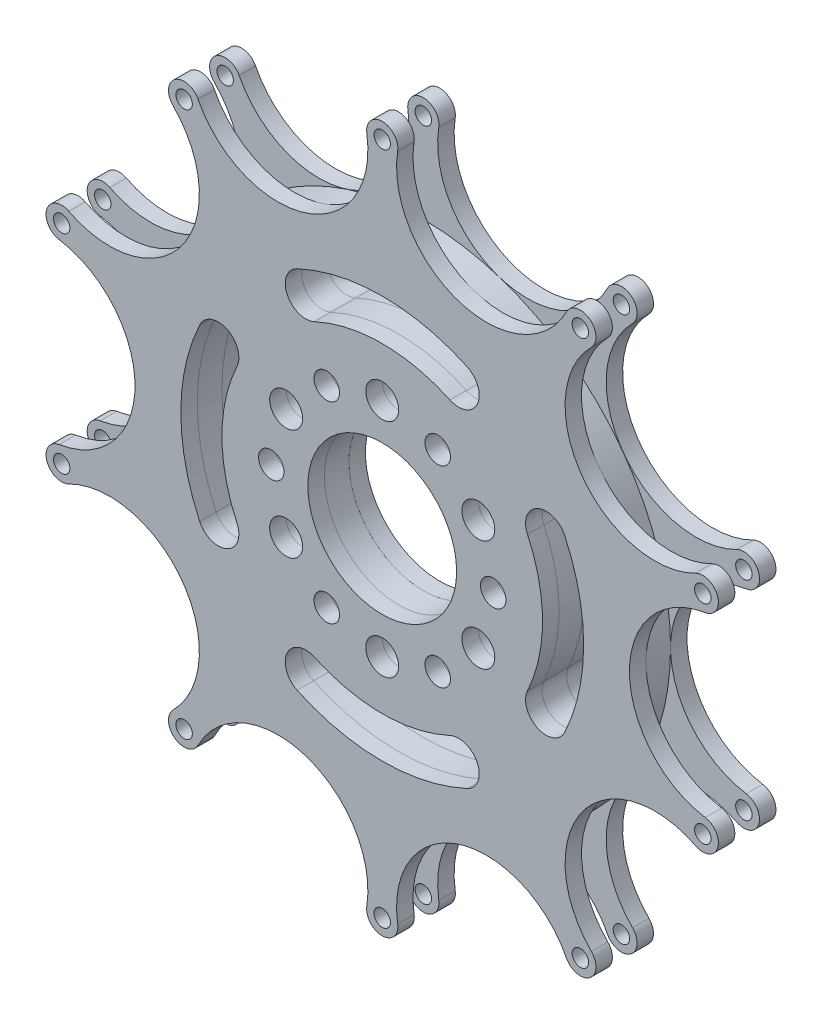
SolidWorks part; units mm, degrees
material "Thornel Mat VMA"
ref_plane "前视基准面" through (0, 0, 0) normal (0, 0, 1) x (1, 0, 0)
ref_plane "上视基准面" through (0, 0, 0) normal (0, 1, 0) x (1, 0, 0)
ref_plane "右视基准面" through (0, 0, 0) normal (1, 0, 0) x (0, 0, -1)
sketch "草图1" plane through (0, 0, 0) normal (0, 0, 1) x (1, 0, 0)
  line L0 (0, 0) -> (0, 41) construction
  circle A0 centre (0, 0) radius 30.0724 construction
  circle A1 centre (0, 0) radius 41 construction
  arc A2 (1.8766, 40.7028) -> (-1.8766, 40.7028) centre (0, 41) ccw
  circle A3 centre (0, 41) radius 1
  arc A4 (1.8766, 40.7028) -> (9.2929, 28.6005) centre (12.6697, 38.9933) ccw
  arc A5 (-1.8766, 40.7028) -> (-9.2929, 28.6005) centre (-12.6697, 38.9933) cw
  circle A6 centre (0, 41) radius 2.5 construction
  arc A7 (25.4427, 31.8262) -> (24.3291, 17.6761) centre (33.1697, 24.0992) ccw
  arc A8 (22.4063, 34.0323) -> (9.2929, 28.6005) centre (12.6697, 38.9933) cw
  arc A9 (25.4427, 31.8262) -> (22.4063, 34.0323) centre (24.0992, 33.1697) ccw
  arc A10 (39.2905, 10.7931) -> (30.0724, 0) centre (41, 0) ccw
  arc A11 (38.1307, 14.3626) -> (24.3291, 17.6761) centre (33.1697, 24.0992) cw
  arc A12 (39.2905, 10.7931) -> (38.1307, 14.3626) centre (38.9933, 12.6697) ccw
  arc A13 (38.1307, -14.3626) -> (24.3291, -17.6761) centre (33.1697, -24.0992) ccw
  arc A14 (39.2905, -10.7931) -> (30.0724, 0) centre (41, 0) cw
  arc A15 (38.1307, -14.3626) -> (39.2905, -10.7931) centre (38.9933, -12.6697) ccw
  arc A16 (22.4063, -34.0323) -> (9.2929, -28.6005) centre (12.6697, -38.9933) ccw
  arc A17 (25.4427, -31.8262) -> (24.3291, -17.6761) centre (33.1697, -24.0992) cw
  arc A18 (22.4063, -34.0323) -> (25.4427, -31.8262) centre (24.0992, -33.1697) ccw
  arc A19 (-1.8766, -40.7028) -> (-9.2929, -28.6005) centre (-12.6697, -38.9933) ccw
  arc A20 (1.8766, -40.7028) -> (9.2929, -28.6005) centre (12.6697, -38.9933) cw
  arc A21 (-1.8766, -40.7028) -> (1.8766, -40.7028) centre (0, -41) ccw
  arc A22 (-25.4427, -31.8262) -> (-24.3291, -17.6761) centre (-33.1697, -24.0992) ccw
  arc A23 (-22.4063, -34.0323) -> (-9.2929, -28.6005) centre (-12.6697, -38.9933) cw
  arc A24 (-25.4427, -31.8262) -> (-22.4063, -34.0323) centre (-24.0992, -33.1697) ccw
  arc A25 (-39.2905, -10.7931) -> (-30.0724, 0) centre (-41, 0) ccw
  arc A26 (-38.1307, -14.3626) -> (-24.3291, -17.6761) centre (-33.1697, -24.0992) cw
  arc A27 (-39.2905, -10.7931) -> (-38.1307, -14.3626) centre (-38.9933, -12.6697) ccw
  arc A28 (-38.1307, 14.3626) -> (-24.3291, 17.6761) centre (-33.1697, 24.0992) ccw
  arc A29 (-39.2905, 10.7931) -> (-30.0724, 0) centre (-41, 0) cw
  arc A30 (-38.1307, 14.3626) -> (-39.2905, 10.7931) centre (-38.9933, 12.6697) ccw
  arc A31 (-22.4063, 34.0323) -> (-9.2929, 28.6005) centre (-12.6697, 38.9933) ccw
  arc A32 (-25.4427, 31.8262) -> (-24.3291, 17.6761) centre (-33.1697, 24.0992) cw
  arc A33 (-22.4063, 34.0323) -> (-25.4427, 31.8262) centre (-24.0992, 33.1697) ccw
  circle A34 centre (-12.6697, 38.9933) radius 9 construction
  circle A36 centre (24.0992, 33.1697) radius 1
  circle A37 centre (38.9933, 12.6697) radius 1
  circle A38 centre (38.9933, -12.6697) radius 1
  circle A39 centre (24.0992, -33.1697) radius 1
  circle A40 centre (0, -41) radius 1
  circle A41 centre (-24.0992, -33.1697) radius 1
  circle A42 centre (-38.9933, -12.6697) radius 1
  circle A43 centre (-38.9933, 12.6697) radius 1
  circle A44 centre (-24.0992, 33.1697) radius 1
  point P78 (0, 0)
  point P88 (0, 0)
  point P98 (0, 0)
  point P107 (0, 0)
  dimension "D1" = 10.9276
  dimension "D2" = 82
  dimension "D3" = 3.8
  dimension "D4" = 2
  dimension "D5" = 5
  dimension "D7" = 60.1447
  dimension "D8" = 18
  dimension "D6" = 10
  dimension "D9" = 10
extrude "凸台-拉伸2" add sketch "草图1" along normal blind 2
sketch "草图2" plane through (0, 0, 2) normal (0, 0, 1) x (1, 0, 0)
  circle A9 centre (0, 0) radius 30.0724 construction
  circle A19 centre (0, 0) radius 30.0724
extrude "凸台-拉伸3" add sketch "草图2" along normal blind 3 separate body
sketch "草图3" plane through (0, 0, 5) normal (0, 0, 1) x (1, 0, 0)
  circle A16 centre (-38.9933, -12.6697) radius 1 construction
  circle A17 centre (-38.9933, 12.6697) radius 1 construction
  circle A18 centre (-24.0992, 33.1697) radius 1 construction
  circle A19 centre (0, 41) radius 1 construction
  arc A20 (-22.4063, 34.0323) -> (-1.8766, 40.7028) centre (-12.6697, 38.9933) ccw
  arc A21 (1.8766, 40.7028) -> (-1.8766, 40.7028) centre (0, 41) ccw
  arc A22 (1.8766, 40.7028) -> (22.4063, 34.0323) centre (12.6697, 38.9933) ccw
  arc A23 (25.4427, 31.8262) -> (22.4063, 34.0323) centre (24.0992, 33.1697) ccw
  arc A24 (25.4427, 31.8262) -> (38.1307, 14.3626) centre (33.1697, 24.0992) ccw
  arc A25 (39.2905, 10.7931) -> (38.1307, 14.3626) centre (38.9933, 12.6697) ccw
  arc A26 (39.2905, 10.7931) -> (39.2905, -10.7931) centre (41, 0) ccw
  arc A27 (38.1307, -14.3626) -> (39.2905, -10.7931) centre (38.9933, -12.6697) ccw
  arc A28 (38.1307, -14.3626) -> (25.4427, -31.8262) centre (33.1697, -24.0992) ccw
  arc A29 (22.4063, -34.0323) -> (25.4427, -31.8262) centre (24.0992, -33.1697) ccw
  arc A30 (22.4063, -34.0323) -> (1.8766, -40.7028) centre (12.6697, -38.9933) ccw
  arc A31 (-1.8766, -40.7028) -> (1.8766, -40.7028) centre (0, -41) ccw
  arc A32 (-1.8766, -40.7028) -> (-22.4063, -34.0323) centre (-12.6697, -38.9933) ccw
  arc A33 (-25.4427, -31.8262) -> (-22.4063, -34.0323) centre (-24.0992, -33.1697) ccw
  arc A34 (-25.4427, -31.8262) -> (-38.1307, -14.3626) centre (-33.1697, -24.0992) ccw
  arc A35 (-39.2905, -10.7931) -> (-38.1307, -14.3626) centre (-38.9933, -12.6697) ccw
  arc A36 (-39.2905, -10.7931) -> (-39.2905, 10.7931) centre (-41, 0) ccw
  arc A37 (-38.1307, 14.3626) -> (-39.2905, 10.7931) centre (-38.9933, 12.6697) ccw
  arc A38 (-38.1307, 14.3626) -> (-25.4427, 31.8262) centre (-33.1697, 24.0992) ccw
  arc A39 (-22.4063, 34.0323) -> (-25.4427, 31.8262) centre (-24.0992, 33.1697) ccw
  arc A40 (-22.4063, 34.0323) -> (-1.8766, 40.7028) centre (-12.6697, 38.9933) ccw
  arc A41 (1.8766, 40.7028) -> (-1.8766, 40.7028) centre (0, 41) ccw
  arc A42 (1.8766, 40.7028) -> (22.4063, 34.0323) centre (12.6697, 38.9933) ccw
  arc A43 (25.4427, 31.8262) -> (22.4063, 34.0323) centre (24.0992, 33.1697) ccw
  arc A44 (25.4427, 31.8262) -> (38.1307, 14.3626) centre (33.1697, 24.0992) ccw
  arc A45 (39.2905, 10.7931) -> (38.1307, 14.3626) centre (38.9933, 12.6697) ccw
  arc A46 (39.2905, 10.7931) -> (39.2905, -10.7931) centre (41, 0) ccw
  arc A47 (38.1307, -14.3626) -> (39.2905, -10.7931) centre (38.9933, -12.6697) ccw
  arc A48 (38.1307, -14.3626) -> (25.4427, -31.8262) centre (33.1697, -24.0992) ccw
  arc A49 (22.4063, -34.0323) -> (25.4427, -31.8262) centre (24.0992, -33.1697) ccw
  arc A50 (22.4063, -34.0323) -> (1.8766, -40.7028) centre (12.6697, -38.9933) ccw
  arc A51 (-1.8766, -40.7028) -> (1.8766, -40.7028) centre (0, -41) ccw
  arc A52 (-1.8766, -40.7028) -> (-22.4063, -34.0323) centre (-12.6697, -38.9933) ccw
  arc A53 (-25.4427, -31.8262) -> (-22.4063, -34.0323) centre (-24.0992, -33.1697) ccw
  arc A54 (-25.4427, -31.8262) -> (-38.1307, -14.3626) centre (-33.1697, -24.0992) ccw
  arc A55 (-39.2905, -10.7931) -> (-38.1307, -14.3626) centre (-38.9933, -12.6697) ccw
  arc A56 (-39.2905, -10.7931) -> (-39.2905, 10.7931) centre (-41, 0) ccw
  arc A57 (-38.1307, 14.3626) -> (-39.2905, 10.7931) centre (-38.9933, 12.6697) ccw
  arc A58 (-38.1307, 14.3626) -> (-25.4427, 31.8262) centre (-33.1697, 24.0992) ccw
  arc A59 (-22.4063, 34.0323) -> (-25.4427, 31.8262) centre (-24.0992, 33.1697) ccw
  circle A60 centre (24.0992, 33.1697) radius 1 construction
  circle A61 centre (38.9933, 12.6697) radius 1 construction
  circle A62 centre (38.9933, -12.6697) radius 1 construction
  circle A63 centre (24.0992, -33.1697) radius 1 construction
  circle A64 centre (0, -41) radius 1 construction
  circle A65 centre (-24.0992, -33.1697) radius 1 construction
  circle A66 centre (-38.9933, -12.6697) radius 1
  circle A67 centre (-38.9933, 12.6697) radius 1
  circle A68 centre (-24.0992, 33.1697) radius 1
  circle A69 centre (0, 41) radius 1
  circle A70 centre (24.0992, 33.1697) radius 1
  circle A71 centre (38.9933, 12.6697) radius 1
  circle A72 centre (38.9933, -12.6697) radius 1
  circle A73 centre (24.0992, -33.1697) radius 1
  circle A74 centre (0, -41) radius 1
  circle A75 centre (-24.0992, -33.1697) radius 1
  dimension "D1" = 0
extrude "凸台-拉伸4" add sketch "草图3" along normal blind 2 separate body
sketch "草图4" plane through (0, 0, 7) normal (0, 0, 1) x (1, 0, 0)
  line L0 (0, 0) -> (41.8998, 0) construction
  line L1 (0, 0) -> (11.6913, 6.75) construction
  line L2 (0, 0) -> (19.9388, -9.2976) construction
  circle A1 centre (0, 0) radius 13.5 construction
  circle A2 centre (13.5, 0) radius 1.55
  circle A4 centre (11.6913, 6.75) radius 2
  circle A5 centre (11.6913, -6.75) radius 2
  circle A6 centre (6.75, -11.6913) radius 1.55
  circle A7 centre (0, -13.5) radius 2
  circle A8 centre (-6.75, -11.6913) radius 1.55
  circle A9 centre (-11.6913, -6.75) radius 2
  circle A10 centre (-13.5, 0) radius 1.55
  circle A11 centre (-11.6913, 6.75) radius 2
  circle A12 centre (-6.75, 11.6913) radius 1.55
  circle A13 centre (0, 13.5) radius 2
  circle A14 centre (6.75, 11.6913) radius 1.55
  circle A15 centre (0, 0) radius 30.0724 construction
  circle A16 centre (0, 0) radius 30.0724 construction
  arc A17 (19.9388, 9.2976) -> (19.9388, -9.2976) centre (0, 0) cw construction
  arc A22 (22.2045, -10.3541) -> (22.2045, 10.3541) centre (0, 0) ccw
  arc A27 (17.673, -8.2411) -> (17.673, 8.2411) centre (0, 0) ccw
  arc A32 (17.673, -8.2411) -> (22.2045, -10.3541) centre (19.9388, -9.2976) ccw
  arc A37 (22.2045, 10.3541) -> (17.673, 8.2411) centre (19.9388, 9.2976) ccw
  arc A42 (9.2976, -19.9388) -> (-9.2976, -19.9388) centre (0, 0) cw construction
  arc A47 (-10.3541, -22.2045) -> (10.3541, -22.2045) centre (0, 0) ccw
  arc A52 (-8.2411, -17.673) -> (8.2411, -17.673) centre (0, 0) ccw
  arc A57 (-8.2411, -17.673) -> (-10.3541, -22.2045) centre (-9.2976, -19.9388) ccw
  arc A58 (10.3541, -22.2045) -> (8.2411, -17.673) centre (9.2976, -19.9388) ccw
  arc A59 (-19.9388, -9.2976) -> (-19.9388, 9.2976) centre (0, 0) cw construction
  arc A60 (-22.2045, 10.3541) -> (-22.2045, -10.3541) centre (0, 0) ccw
  arc A61 (-17.673, 8.2411) -> (-17.673, -8.2411) centre (0, 0) ccw
  arc A62 (-17.673, 8.2411) -> (-22.2045, 10.3541) centre (-19.9388, 9.2976) ccw
  arc A63 (-22.2045, -10.3541) -> (-17.673, -8.2411) centre (-19.9388, -9.2976) ccw
  arc A64 (-9.2976, 19.9388) -> (9.2976, 19.9388) centre (0, 0) cw construction
  arc A65 (10.3541, 22.2045) -> (-10.3541, 22.2045) centre (0, 0) ccw
  arc A66 (8.2411, 17.673) -> (-8.2411, 17.673) centre (0, 0) ccw
  arc A67 (8.2411, 17.673) -> (10.3541, 22.2045) centre (9.2976, 19.9388) ccw
  arc A68 (-10.3541, 22.2045) -> (-8.2411, 17.673) centre (-9.2976, 19.9388) ccw
  point P1 (22, 0)
  point P32 (0, 0)
  point P43 (0, -22)
  point P50 (-22, 0)
  point P57 (0, 22)
  point P64 (0, 0)
  point P72 (17.6777, 17.6777)
  point P79 (0, 18.5)
  point P93 (18.5, 0)
  point P97 (0, 0)
  point P98 (-17.6777, 17.6777)
  dimension "D1" = 2.5
  dimension "D2" = 27
  dimension "D4" = 3.1
  dimension "D5" = 4
  dimension "D6" = 6
  dimension "D7" = 22
  dimension "D3" = 30
  dimension "D8" = 25
  dimension "D9" = 4
extrude "切除-拉伸1" cut sketch "草图4" against normal blind 10
sketch "草图6" plane through (0, 0, 7) normal (0, 0, 1) x (1, 0, 0)
  circle A0 centre (0, 0) radius 9.05
  dimension "D1" = 18.1
extrude "切除-拉伸3" cut sketch "草图6" against normal through all both and the other way through all
